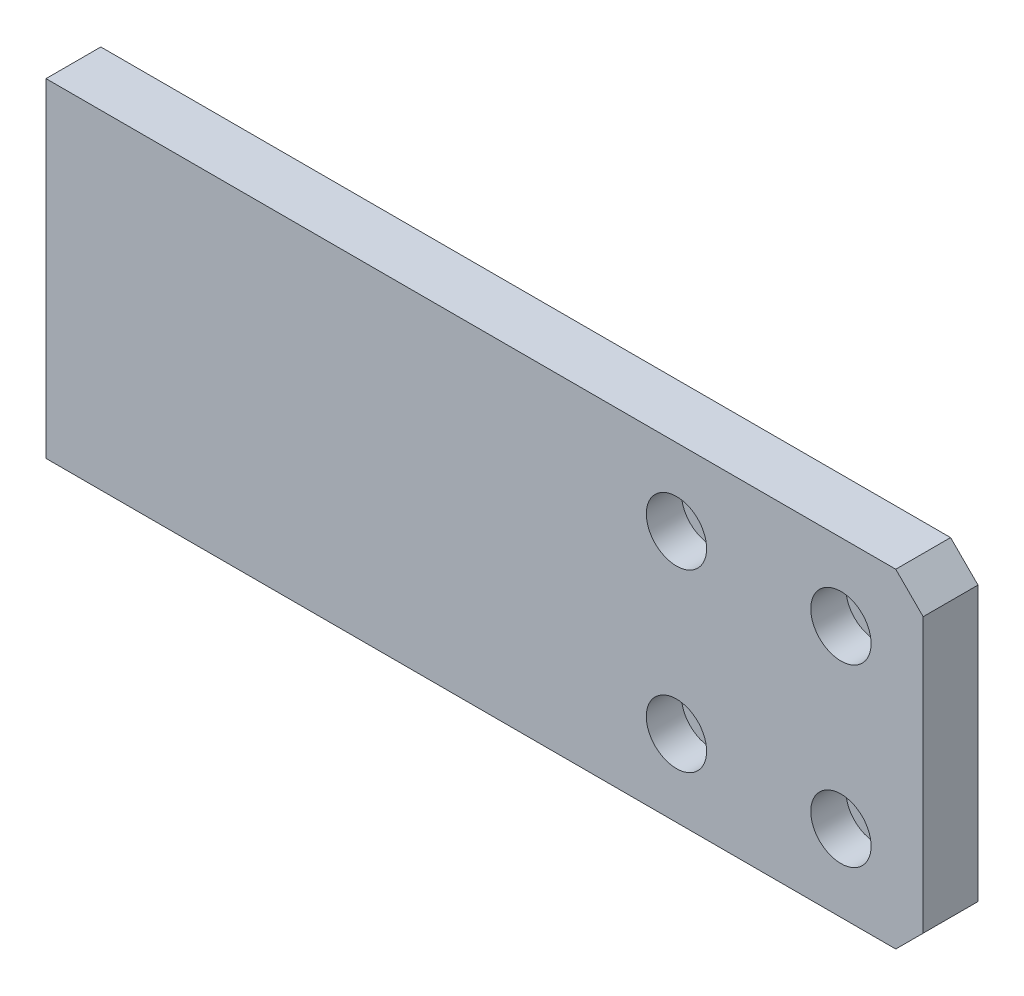
from build123d import *

# Parameters (mm, degrees)
SKETCH1_W                                           = 160
SKETCH1_H                                           = 60
BOSS_EXTRUDE1_DEPTH                                 = 5
CBORE_FOR_M6_HEX_SOCKET_HEAD_CAP_SCREW1_D           = 6.6
CBORE_FOR_M6_HEX_SOCKET_HEAD_CAP_SCREW1_CBORE_D     = 11
CBORE_FOR_M6_HEX_SOCKET_HEAD_CAP_SCREW1_CBORE_DEPTH = 6.4
CHAMFER1_SIZE                                       = 5
M6_TAPPED_HOLE1_D                                   = 5
M6_TAPPED_HOLE1_DEPTH                               = 11
M6_TAPPED_HOLE1_TIP                                 = 1.502151548


with BuildPart() as part:
    # Sketch1 → Boss-Extrude1 (new, symmetric)
    with BuildSketch(Plane.XY):
        Rectangle(SKETCH1_W, SKETCH1_H)
    extrude(amount=BOSS_EXTRUDE1_DEPTH, both=True)

    # CBORE for M6 Hex Socket Head Cap Screw1 (through all)
    with Locations(Plane.XY.offset(5)):
        with Locations((35, -16), (65, -16), (65, 16), (35, 16)):
            CounterBoreHole(CBORE_FOR_M6_HEX_SOCKET_HEAD_CAP_SCREW1_D / 2, CBORE_FOR_M6_HEX_SOCKET_HEAD_CAP_SCREW1_CBORE_D / 2, CBORE_FOR_M6_HEX_SOCKET_HEAD_CAP_SCREW1_CBORE_DEPTH)

    # Chamfer1
    chamfer1_edges = [part.edges().sort_by_distance(p)[0] for p in [
        (80, -30, 0),
        (80, 30, 0),
    ]]
    chamfer(chamfer1_edges, length=CHAMFER1_SIZE)

    # M6 Tapped Hole1
    with Locations(Plane.ZY.offset(80)):
        with Locations((0, 18), (0, 0), (0, -18)):
            Hole(M6_TAPPED_HOLE1_D / 2, depth=M6_TAPPED_HOLE1_DEPTH)
            with Locations((0, 0, -(M6_TAPPED_HOLE1_DEPTH + M6_TAPPED_HOLE1_TIP / 2))):  # 118° drill point
                Cone(0, M6_TAPPED_HOLE1_D / 2, M6_TAPPED_HOLE1_TIP, mode=Mode.SUBTRACT)


solid = part.part
